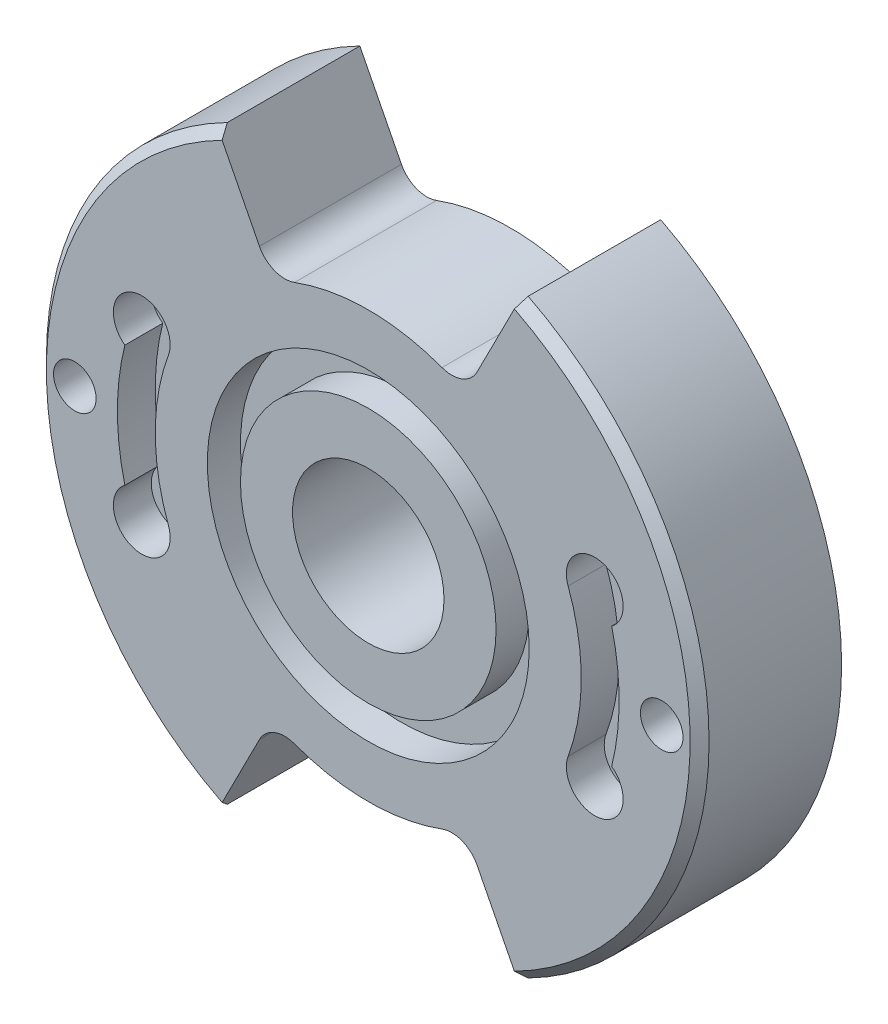
SolidWorks part; units mm, degrees
ref_plane "前视基准面" through (0, 0, 0) normal (0, 0, 1) x (1, 0, 0)
ref_plane "上视基准面" through (0, 0, 0) normal (0, 1, 0) x (1, 0, 0)
ref_plane "右视基准面" through (0, 0, 0) normal (1, 0, 0) x (0, 0, -1)
sketch "草图1" plane through (0, 0, 0) normal (0, 0, 1) x (1, 0, 0)
  circle A0 centre (0, 0) radius 35
extrude "凸台-拉伸1" add sketch "草图1" along normal blind 15
sketch "草图2" plane through (0, 0, 15) normal (0, 0, 1) x (1, 0, 0)
  line L0 (0, 37.8819) -> (0, 0) construction
  line L1 (0, 0) -> (17.5352, 34.4148) construction
  line L2 (0, 0) -> (-17.9291, 35.1878) construction
  line L3 (-16.6707, 32.718) -> (-10.2148, 20.0476)
  line L4 (16.6707, 32.718) -> (10.2148, 20.0476)
  arc A0 (10.2148, 20.0476) -> (-10.2148, 20.0476) centre (0, 0) ccw
  arc A1 (16.6707, 32.718) -> (-16.6707, 32.718) centre (0, 0) ccw
  dimension "D1" = 27
  dimension "D2" = 27
extrude "切除-拉伸1" cut sketch "草图2" against normal blind 15
fillet "圆角1" radius 3 2 edges at (10.2148, 20.0476, 7.5) (-10.2148, 20.0476, 7.5)
mirror "镜向1" about plane through (0, 0, 0) normal (0, 1, 0) of "切除-拉伸1", "圆角1"
sketch "草图3" plane through (0, 0, 15) normal (0, 0, 1) x (1, 0, 0)
  circle A0 centre (0, 0) radius 17
  circle A1 centre (0, 0) radius 13.5
extrude "切除-拉伸2" cut sketch "草图3" against normal blind 3.5
sketch "草图4" plane through (0, 0, 15) normal (0, 0, 1) x (1, 0, 0)
  line L0 (0, 0) -> (40.662, 0) construction
  line L1 (0, 0) -> (35.5918, 18.1349) construction
  line L2 (0, 0) -> (33.7213, -17.1818) construction
  arc A0 (21.1102, 7.7853) -> (21.1102, -7.7853) centre (0, 0) cw
  arc A1 (25.7121, 6.4138) -> (25.7121, -6.4138) centre (0, 0) cw
  arc A2 (21.1102, -7.7853) -> (25.7121, -6.4138) centre (23.9249, -8.8233) ccw
  arc A3 (25.7121, 6.4138) -> (21.1102, 7.7853) centre (23.9249, 8.8233) ccw
  dimension "D3" = 26.5
  dimension "D4" = 22.5
  dimension "D1" = 27
  dimension "D2" = 27
extrude "切除-拉伸3" cut sketch "草图4" against normal blind 4
mirror "镜向2" about plane through (0, 0, 0) normal (1, 0, 0) of "切除-拉伸3"
sketch "草图5" plane through (0, 0, 15) normal (0, 0, 1) x (1, 0, 0)
  circle A0 centre (0, 0) radius 8
extrude "切除-拉伸4" cut sketch "草图5" against normal through all
sketch "草图6" plane through (0, 0, 15) normal (0, 0, 1) x (1, 0, 0)
  line L0 (-31, 0) -> (31, 0) construction
  circle A0 centre (-31, 0) radius 2.25
  circle A1 centre (31, 0) radius 2.25
  dimension "D1" = 31
  dimension "D2" = 31
extrude "切除-拉伸5" cut sketch "草图6" against normal through all
chamfer "倒角1" distance 1 angle 45 2 edges at (35, 0, 15) (-35, 0, 15)
